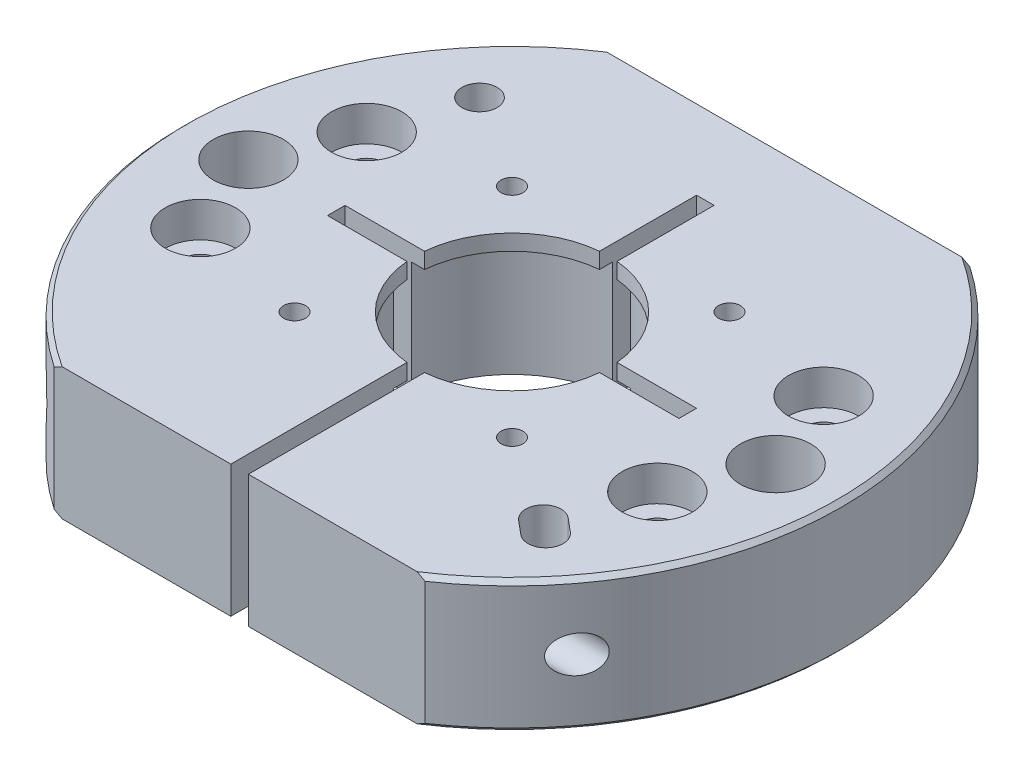
SolidWorks part; units mm, degrees
ref_plane "Front Plane" through (0, 0, 0) normal (0, 0, 1) x (1, 0, 0)
ref_plane "Top Plane" through (0, 0, 0) normal (0, 1, 0) x (1, 0, 0)
ref_plane "Right Plane" through (0, 0, 0) normal (1, 0, 0) x (0, 0, -1)
sketch "Sketch1" plane through (0, 0, 0) normal (0, 1, 0) x (1, 0, 0)
  circle A0 centre (0, 0) radius 37.5
  circle A1 centre (0, 0) radius 12.5
  dimension "D1" = 25
  dimension "D2" = 75
extrude "Boss-Extrude1" add sketch "Sketch1" along normal blind 15
sketch "Sketch2" plane through (0, 15, 0) normal (0, 1, 0) x (1, 0, 0)
  line L0 (0, 0) -> (-50000, 0) construction
  line L1 (-25.7045, 9.3557) -> (46958.9265, -17091.6515) construction
  line L2 (0, 0) -> (0, -50000) construction
  circle A0 centre (26, -9.4632) radius 4
  circle A1 centre (-26, 9.4632) radius 4
  circle A2 centre (-26, -9.4632) radius 4
  circle A3 centre (26, 9.4632) radius 4
  dimension "D1" = 20
  dimension "D2" = 8
  dimension "D3" = 52
extrude "Cut-Extrude1" cut sketch "Sketch2" against normal blind 4
sketch "Sketch3" plane through (0, 15, 0) normal (0, 1, 0) x (1, 0, 0)
  circle A0 centre (-26, 9.4632) radius 2
  circle A1 centre (-26, -9.4632) radius 2
  circle A2 centre (26, 9.4632) radius 2
  circle A3 centre (26, -9.4632) radius 2
  dimension "D1" = 4
  dimension "D2" = 4
  dimension "D3" = 4
extrude "Cut-Extrude2" cut sketch "Sketch3" against normal through all
sketch "Sketch4" plane through (0, 15, 0) normal (0, 1, 0) x (1, 0, 0)
  line L0 (0, 0) -> (0, -50000) construction
  line L1 (0, 0) -> (-50000, 0) construction
  line L3 (-20, 1) -> (20, 1)
  line L4 (-20, 1) -> (-20, -1)
  line L5 (-20, -1) -> (20, -1)
  line L6 (20, 1) -> (20, -1)
  line L7 (-20, 1) -> (20, -1) construction
  line L8 (-20, -1) -> (20, 1) construction
  point P5 (0, 0)
  dimension "D1" = 2
  dimension "D2" = 40
extrude "Cut-Extrude3" cut sketch "Sketch4" against normal blind 16
sketch "Sketch5" plane through (0, 15, 0) normal (0, 1, 0) x (1, 0, 0)
  line L0 (0, 0) -> (0, 50000) construction
  line L1 (0, 0) -> (-50000, 0) construction
  line L2 (-1, -45) -> (1, -45)
  line L3 (-1, -45) -> (-1, 22)
  line L4 (-1, 22) -> (1, 22)
  line L5 (1, -45) -> (1, 22)
  line L6 (-1, -45) -> (1, 22) construction
  line L7 (-1, 22) -> (1, -45) construction
  point P3 (0, -11.5)
  dimension "D1" = 2
  dimension "D2" = 22
  dimension "D3" = 45
extrude "Cut-Extrude4" cut sketch "Sketch5" against normal blind 16
chamfer "Chamfer1" distance 0.5 angle 45 2 edges at (0, 0, -37.5) (0, 15, -37.5)
sketch "Sketch6" plane through (0, 0, 0) normal (1, 0, 0) x (0, 0, -1)
  line L0 (-27.4818, 7.5) -> (49972.5182, 7.5) construction
  line L1 (-37.4867, 14.5) -> (-37.4867, 0.5) construction
  circle A0 centre (-22.5, 7.5) radius 2.75
  point P4 (-37.4867, 7.5)
  dimension "D1" = 5.5
  dimension "D2" = 22.5
extrude "Cut-Extrude5" cut sketch "Sketch6" against normal blind 27
ref_plane "Plane1" through (-8.5, 0, 0) normal (1, 0, 0) x (0, 0, -1)
sketch "Sketch7" plane through (-8.5, 0, 0) normal (1, 0, 0) x (0, 0, -1)
  circle A0 centre (-22.5, 7.5) radius 5.5
  dimension "D1" = 11
extrude "Cut-Extrude6" cut sketch "Sketch7" against normal blind 27
sketch "Sketch8" plane through (1, 0, 0) normal (-1, 0, 0) x (0, 0, 1)
  circle A0 centre (22.5, 7.5) radius 0.5428
extrude "Cut-Extrude7" cut sketch "Sketch8" against normal blind 27
hole_wizard "M5 Tapped Hole1" positions "3DSketch1" profile "Sketch9" tap size "M5" standard "Gb"
sketch3d "3DSketch1"
  line L0 (28, 7.5, 22.5) -> (1, 7.5, 22.5) construction
  point P0 (1, 7.5, 22.5)
cosmetic thread "Hole Thread 1" parameters "D2"=5
sketch "Sketch9" plane through (1, 7.5, 22.5) normal (0, 1, 0) x (0, 0, 1)
  line L0 (0, 0) -> (0, 36.5)
  line L1 (0, 36.5) -> (2.1, 36.5)
  line L2 (2.1, 36.5) -> (2.1, 0)
  line L5 (2.1, 0) -> (0, 0)
  line L11 (0, -6.35) -> (0, 107.95) construction
  dimension "通孔螺纹孔钻头直径" = 4.2
  dimension "通孔螺纹孔钻头深度" = 36.5
sketch "Sketch10" plane through (0, 15, 0) normal (0, 1, 0) x (1, 0, 0)
  line L0 (0, 0) -> (0, 50000) construction
  line L1 (0, 0) -> (50000, 0) construction
  circle A0 centre (-30, 0) radius 4
  circle A1 centre (30, 0) radius 4
  dimension "D1" = 60
  dimension "D2" = 8
extrude "Cut-Extrude8" cut sketch "Sketch10" against normal through all
sketch "Sketch11" plane through (0, 15, 0) normal (0, 1, 0) x (1, 0, 0)
  line L0 (0, 0) -> (50000, 0) construction
  line L1 (0, 0) -> (0, 50000) construction
  line L2 (-35, -31) -> (35, -31)
  line L3 (-35, 44) -> (35, 44)
  line L4 (-35, 44) -> (-35, 31)
  line L5 (-35, 31) -> (35, 31)
  line L6 (35, 44) -> (35, 31)
  line L7 (-35, 44) -> (35, 31) construction
  line L8 (-35, 31) -> (35, 44) construction
  line L9 (35, -44) -> (35, -31)
  line L10 (-35, -44) -> (35, -44)
  line L11 (-35, -44) -> (-35, -31)
  line L12 (-35, -31) -> (35, -44) construction
  line L13 (-35, -44) -> (35, -31) construction
  arc A0 (1, -37.4867) -> (-1, -37.4867) centre (0, 0) ccw construction
  point P5 (0, 37.5)
  point P17 (0, -37.5)
  dimension "D1" = 62
  dimension "D2" = 70
extrude "Cut-Extrude9" cut sketch "Sketch11" against normal through all
sketch "Sketch16" plane through (0, 0, 0) normal (0, -1, 0) x (1, 0, 0)
  line L0 (0, 0) -> (0, -50000) construction
  line L1 (0, 0) -> (-38302.2222, -32139.3805) construction
  line L2 (23.7474, 19.9264) -> (22.2153, 18.6408) construction
  line L3 (25.033, 18.3943) -> (23.5009, 17.1088)
  line L4 (22.4618, 21.4585) -> (20.9297, 20.1729)
  circle A0 centre (0, 0) radius 30 construction
  arc A1 (25.033, 18.3943) -> (22.4618, 21.4585) centre (23.7474, 19.9264) ccw
  circle A2 centre (-22.9813, -19.2836) radius 2
  arc A3 (20.9297, 20.1729) -> (23.5009, 17.1088) centre (22.2153, 18.6408) ccw
  point P11 (22.9813, 19.2836)
  dimension "D2" = 60
  dimension "D3" = 4
  dimension "D1" = 50
  dimension "D4" = 2
  dimension "D5" = 4
extrude "Cut-Extrude11" cut sketch "Sketch16" against normal through all
sketch "Sketch17" plane through (0, 15, 0) normal (0, 1, 0) x (1, 0, 0)
  line L0 (1, 12.4599) -> (1, 10.9545)
  line L1 (-1, 12.4599) -> (-1, 10.9545)
  line L2 (12.4599, 1) -> (10.9545, 1)
  line L3 (12.4599, -1) -> (10.9545, -1)
  line L4 (-12.4599, 1) -> (-10.9545, 1)
  line L5 (-12.4599, -1) -> (-10.9545, -1)
  line L6 (1, -12.4599) -> (1, -10.9545)
  line L7 (-1, -12.4599) -> (-1, -10.9545)
  arc A0 (10.9545, 1) -> (1, 10.9545) centre (0, 0) ccw
  arc A1 (-1, 10.9545) -> (-10.9545, 1) centre (0, 0) ccw
  arc A2 (-10.9545, -1) -> (-1, -10.9545) centre (0, 0) ccw
  arc A3 (1, -10.9545) -> (10.9545, -1) centre (0, 0) ccw
  arc A4 (12.4599, 1) -> (1, 12.4599) centre (0, 0) ccw construction
  arc A5 (-1, 12.4599) -> (-12.4599, 1) centre (0, 0) ccw construction
  arc A6 (-12.4599, -1) -> (-1, -12.4599) centre (0, 0) ccw construction
  arc A7 (1, -12.4599) -> (12.4599, -1) centre (0, 0) ccw construction
  arc A8 (12.4599, 1) -> (1, 12.4599) centre (0, 0) ccw
  arc A9 (-1, 12.4599) -> (-12.4599, 1) centre (0, 0) ccw
  arc A10 (-12.4599, -1) -> (-1, -12.4599) centre (0, 0) ccw
  arc A11 (1, -12.4599) -> (12.4599, -1) centre (0, 0) ccw
  dimension "D1" = 22
extrude "Boss-Extrude2" add sketch "Sketch17" against normal blind 1.8
sketch "Sketch19" plane through (0, 15, 0) normal (0, 1, 0) x (1, 0, 0)
  line L0 (0, 0) -> (0, 50000) construction
  line L1 (0, 0) -> (50000, 0) construction
  line L2 (0, 0) -> (-35355.3391, 35355.3391) construction
  circle A0 centre (0, 0) radius 17.5 construction
  circle A1 centre (-12.3744, 12.3744) radius 1
  dimension "D1" = 35
  dimension "D2" = 45
  dimension "D3" = 2
extrude "Cut-Extrude12" cut sketch "Sketch19" against normal blind 5
hole_wizard "M3 Tapped Hole2" positions "3DSketch3" profile "Sketch20" tap size "M3" standard "Gb"
sketch3d "3DSketch3"
  line L0 (-12.3744, 10, -12.3744) -> (-12.3744, 15, -12.3744) construction
  point P0 (-12.3744, 15, -12.3744)
sketch "Sketch20" plane through (-12.3744, 15, -12.3744) normal (1, 0, 0) x (0, 0, 1)
  line L0 (0, 0) -> (0, 7.2511)
  line L1 (0, 7.2511) -> (1.25, 6.5)
  line L2 (1.25, 6.5) -> (1.25, 0)
  line L5 (1.25, 0) -> (0, 0)
  line L10 (0, 7.2511) -> (-1.25, 6.5) construction
  line L11 (0, -6.35) -> (0, 107.95) construction
  dimension "螺纹孔钻头直径" = 2.5
  dimension "螺纹孔钻头深度" = 6.5
  dimension "导头角度" = 118
cosmetic thread "Hole Thread 3" parameters "D1"=5, "D2"=3
pattern_circular "CirPattern2" count 4 every 90 about axis through (0, 0, 0) along (0, 1, 0) of "M3 Tapped Hole2"
